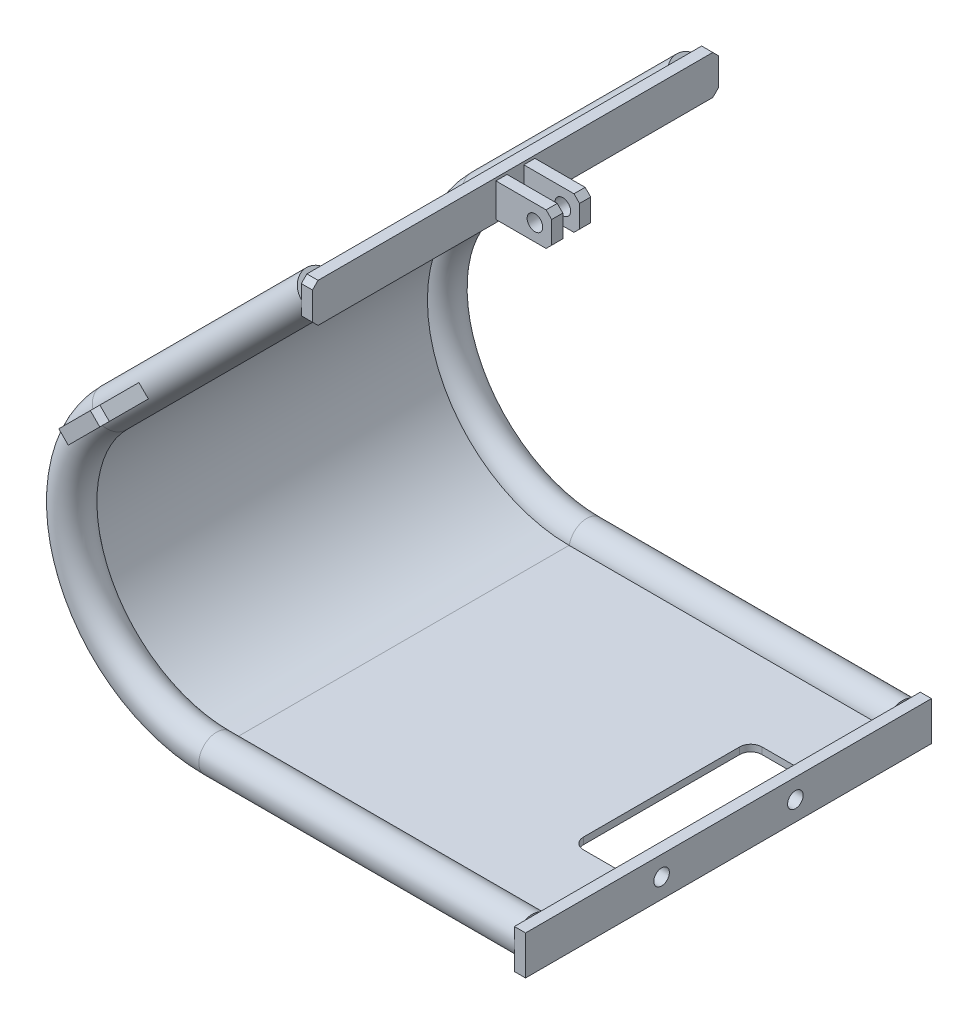
from build123d import *

# Parameters (mm, degrees)
SKETCH_2_R               = 16
SKETCH_2_R_2             = 11
CUT_EXTRUDE_1_DEPTH      = 485.515318427
CUT_EXTRUDE_1_DEPTH_BACK = 485.515318427
SKETCH_4_W               = 55.642342567
SKETCH_4_H               = 67.933254927
EXTRUDE_START            = 16
EXTRUDE_2_DEPTH          = 300
SKETCH_7_R               = 16
SKETCH_7_R_2             = 11
SKETCH_9_W               = 513.497861872
SKETCH_9_H               = 78.296499381
CUT_EXTRUDE_2_DEPTH      = 597.324654745
SKETCH_10_W              = 364
SKETCH_10_H              = 35
EXTRUDE_2_2_DEPTH        = 10
SKETCH_11_W              = 364
SKETCH_11_H              = 35
EXTRUDE_4_DEPTH          = 10
CHAMFER_1_SIZE           = 5
CUT_EXTRUDE_4_DEPTH      = 596.26467125
SKETCH_14_R              = 7
CUT_EXTRUDE_5_DEPTH      = 10
SKETCH_15_W              = 10
SKETCH_15_H              = 30
EXTRUDE_5_DEPTH          = 50
EXTRUDE_5_2_DEPTH        = 50
CHAMFER_2_SIZE           = 5
CHAMFER_3_SIZE           = 5
SKETCH_16_R              = 7
CUT_EXTRUDE_6_DEPTH      = 528.366607347
SKETCH_18_W              = 50
SKETCH_18_H              = 40
SKETCH_18_R              = 7
EXTRUDE_6_DEPTH          = 6
EXTRUDE_6_2_DEPTH        = 6
CHAMFER_4_SIZE           = 5
CHAMFER_5_SIZE           = 5


with BuildPart() as part:
    # 扫描1: sweep along a path in 草图1
    with BuildLine(Plane.XY) as sweep_1_path:
        Line((0, 0), (-183.847763109, -183.847763109))
        ThreePointArc((-183.847763109, -183.847763109), (-212.028220781, -325.52049087), (-91.923881554, -405.771644663))
        Line((-91.923881554, -405.771644663), (191.076118446, -405.771644663))
    # 草图2 → 扫描1 (sweep)
    with BuildSketch(Plane(origin=(191.076118446, 0, 0), x_dir=(0, 0, -1), z_dir=(1, 0, 0))):
        with Locations((0, -405.771644663)):
            Circle(SKETCH_2_R)
        with Locations((0, -405.771644663)):
            Circle(SKETCH_2_R_2, mode=Mode.SUBTRACT)
    sweep(path=sweep_1_path.line)

    # 草图4 → 切除-拉伸1 (cut, two sides: drawn at the far end of the back side and taken through both)
    with BuildSketch(Plane.XY.offset(-CUT_EXTRUDE_1_DEPTH_BACK)):
        with Locations((27.821171284, -33.966627464)):
            Rectangle(SKETCH_4_W, SKETCH_4_H)
    extrude(amount=CUT_EXTRUDE_1_DEPTH + CUT_EXTRUDE_1_DEPTH_BACK, mode=Mode.SUBTRACT)


with BuildPart() as body_2:
    # 草图6 → Extrude 2 (new body)
    with BuildSketch(Plane.XY.offset(EXTRUDE_START)):
        with BuildLine():
            Line((-2.121320344, 2.121320344), (-185.969083452, -181.726442765))
            ThreePointArc((-185.969083452, -181.726442765), (-214.799859378, -326.668541167), (-91.923881554, -408.771644663))
            Line((-91.923881554, -408.771644663), (191.076118446, -408.771644663))
            Line((191.076118446, -408.771644663), (191.076118446, -402.771644663))
            Line((191.076118446, -402.771644663), (-91.923881554, -402.771644663))
            ThreePointArc((-91.923881554, -402.771644663), (-209.256582183, -324.372440573), (-181.726442765, -185.969083452))
            Line((-181.726442765, -185.969083452), (2.121320344, -2.121320344))
            Line((2.121320344, -2.121320344), (-2.121320344, 2.121320344))
        make_face()
    extrude(amount=EXTRUDE_2_DEPTH)


with BuildPart() as body_3:
    # 扫描2: sweep along a path in 草图8
    with BuildLine(Plane.XY.offset(332)) as sweep_2_path:
        Line((0, 0), (-183.847763109, -183.847763109))
        ThreePointArc((-183.847763109, -183.847763109), (-212.028220781, -325.52049087), (-91.923881554, -405.771644663))
        Line((-91.923881554, -405.771644663), (191.076118446, -405.771644663))
    # 草图7 → 扫描2 (sweep)
    with BuildSketch(Plane(origin=(191.076118446, 0, 0), x_dir=(0, 0, -1), z_dir=(1, 0, 0))):
        with Locations((-332, -405.771644663)):
            Circle(SKETCH_7_R)
        with Locations((-332, -405.771644663)):
            Circle(SKETCH_7_R_2, mode=Mode.SUBTRACT)
    sweep(path=sweep_2_path.line)


with BuildPart() as cut_extrude_2_tool:
    # 草图9 → 切除-拉伸2 (new, through all)
    with BuildSketch(Plane(origin=(0, 0, 0), x_dir=(0, 0, -1), z_dir=(1, 0, 0))):
        with Locations((-166, -2.121320344)):
            Rectangle(SKETCH_9_W, SKETCH_9_H)
    extrude(amount=CUT_EXTRUDE_2_DEPTH)


with BuildPart() as body_2_1:
    add(body_2.part)

    # 切除-拉伸2: cut by cut_extrude_2_tool
    add(cut_extrude_2_tool.part, mode=Mode.SUBTRACT)

    # 草图13 → 切除-拉伸4 (cut, through all)
    with BuildSketch(Plane(origin=(0, -402.771644663, 0), x_dir=(1, 0, 0), z_dir=(0, 1, 0))):
        with BuildLine():
            Line((151.076118446, -246), (191.076118446, -246))
            Line((191.076118446, -246), (191.076118446, -86))
            Line((191.076118446, -86), (151.076118446, -86))
            ThreePointArc((151.076118446, -86), (144.005050634, -88.928932188), (141.076118446, -96))
            Line((141.076118446, -96), (141.076118446, -236))
            ThreePointArc((141.076118446, -236), (144.005050634, -243.071067812), (151.076118446, -246))
        make_face()
    extrude(amount=-CUT_EXTRUDE_4_DEPTH, mode=Mode.SUBTRACT)


with BuildPart() as body_3_1:
    add(body_3.part)

    # 切除-拉伸2: cut by cut_extrude_2_tool
    add(cut_extrude_2_tool.part, mode=Mode.SUBTRACT)


with BuildPart() as body_4:
    # 草图10 → Extrude 2 2 (new body)
    with BuildSketch(Plane(origin=(0, 0, 0), x_dir=(0, 0, -1), z_dir=(1, 0, 0))):
        with Locations((-166, 0)):
            Rectangle(SKETCH_10_W, SKETCH_10_H)
    extrude(amount=EXTRUDE_2_2_DEPTH)

    # 倒角1
    chamfer_1_edges = [body_4.edges().sort_by_distance(p)[0] for p in [
        (5, -17.5, -16),
        (5, -17.5, 348),
        (5, 17.5, 348),
        (5, 17.5, -16),
    ]]
    chamfer(chamfer_1_edges, length=CHAMFER_1_SIZE)


with BuildPart() as body_5:
    # 草图11 → 凸台-拉伸4 (new body)
    with BuildSketch(Plane(origin=(191.076118446, 0, 0), x_dir=(0, 0, -1), z_dir=(1, 0, 0))):
        with Locations((-166, -408.771644663)):
            Rectangle(SKETCH_11_W, SKETCH_11_H)
    extrude(amount=EXTRUDE_4_DEPTH)

    # 草图14 → 切除-拉伸5 (cut)
    with BuildSketch(Plane(origin=(201.076118446, 0, 0), x_dir=(0, 0, -1), z_dir=(1, 0, 0))):
        with Locations((-106, -408.771644663)):
            Circle(SKETCH_14_R)
        with Locations((-226, -408.771644663)):
            Circle(SKETCH_14_R)
    extrude(amount=-CUT_EXTRUDE_5_DEPTH, mode=Mode.SUBTRACT)


with BuildPart() as body_6:
    # 草图15 → 凸台-拉伸5 (new body)
    with BuildSketch(Plane(origin=(10, 0, 0), x_dir=(0, 0, -1), z_dir=(1, 0, 0))):
        with Locations((-178.5, 0)):
            Rectangle(SKETCH_15_W, SKETCH_15_H)
    extrude(amount=EXTRUDE_5_DEPTH)

    # 倒角2
    chamfer_2_edges = [body_6.edges().sort_by_distance(p)[0] for p in [
        (60, -15, 178.5),
        (60, 15, 178.5),
    ]]
    chamfer(chamfer_2_edges, length=CHAMFER_2_SIZE)


with BuildPart() as body_7:
    # 草图15 → Extrude 5 2 (new body)
    with BuildSketch(Plane(origin=(10, 0, 0), x_dir=(0, 0, -1), z_dir=(1, 0, 0))):
        with Locations((-153.5, 0)):
            Rectangle(SKETCH_15_W, SKETCH_15_H)
    extrude(amount=EXTRUDE_5_2_DEPTH)

    # 倒角3
    chamfer_3_edges = [body_7.edges().sort_by_distance(p)[0] for p in [
        (60, -15, 153.5),
        (60, 15, 153.5),
    ]]
    chamfer(chamfer_3_edges, length=CHAMFER_3_SIZE)


with BuildPart() as cut_extrude_6_tool:
    # 草图16 → 切除-拉伸6 (new, through all)
    with BuildSketch(Plane.XY.offset(183.5)):
        with Locations((45, 0)):
            Circle(SKETCH_16_R)
    extrude(amount=-CUT_EXTRUDE_6_DEPTH)


with BuildPart() as body_6_1:
    add(body_6.part)

    # 切除-拉伸6: cut by cut_extrude_6_tool
    add(cut_extrude_6_tool.part, mode=Mode.SUBTRACT)


with BuildPart() as body_7_1:
    add(body_7.part)

    # 切除-拉伸6: cut by cut_extrude_6_tool
    add(cut_extrude_6_tool.part, mode=Mode.SUBTRACT)


with BuildPart() as body_8:
    # 草图18 → 凸台-拉伸6 (new, symmetric)
    with BuildSketch(Plane(origin=(0, 0, 0), x_dir=(0.7071067811865511, 0.7071067811865439, 0), z_dir=(-0.7071067811865439, 0.7071067811865511, 0))):
        with Locations((-225, 36)):
            Rectangle(SKETCH_18_W, SKETCH_18_H)
        with Locations(Location((-225, 41, 0), (0, 0, 180))):
            Circle(SKETCH_18_R, mode=Mode.SUBTRACT)
    extrude(amount=EXTRUDE_6_DEPTH, both=True)

    # 倒角4
    chamfer_4_edges = [body_8.edges().sort_by_distance(p)[0] for p in [
        (-176.776695297, -176.776695297, -56),
        (-141.421356237, -141.421356237, -56),
    ]]
    chamfer(chamfer_4_edges, length=CHAMFER_4_SIZE)


with BuildPart() as body_9:
    # 草图18 → Extrude 6 2 (new, symmetric)
    with BuildSketch(Plane(origin=(0, 0, 0), x_dir=(0.7071067811865511, 0.7071067811865439, 0), z_dir=(-0.7071067811865439, 0.7071067811865511, 0))):
        with Locations((-225, -368)):
            Rectangle(SKETCH_18_W, SKETCH_18_H)
        with Locations((-225, -373)):
            Circle(SKETCH_18_R, mode=Mode.SUBTRACT)
    extrude(amount=EXTRUDE_6_2_DEPTH, both=True)

    # 倒角5
    chamfer_5_edges = [body_9.edges().sort_by_distance(p)[0] for p in [
        (-141.421356237, -141.421356237, 388),
        (-176.776695297, -176.776695297, 388),
    ]]
    chamfer(chamfer_5_edges, length=CHAMFER_5_SIZE)


solid = Compound([part.part, body_2_1.part, body_3_1.part, body_4.part, body_5.part, body_6_1.part, body_7_1.part, body_8.part, body_9.part])
